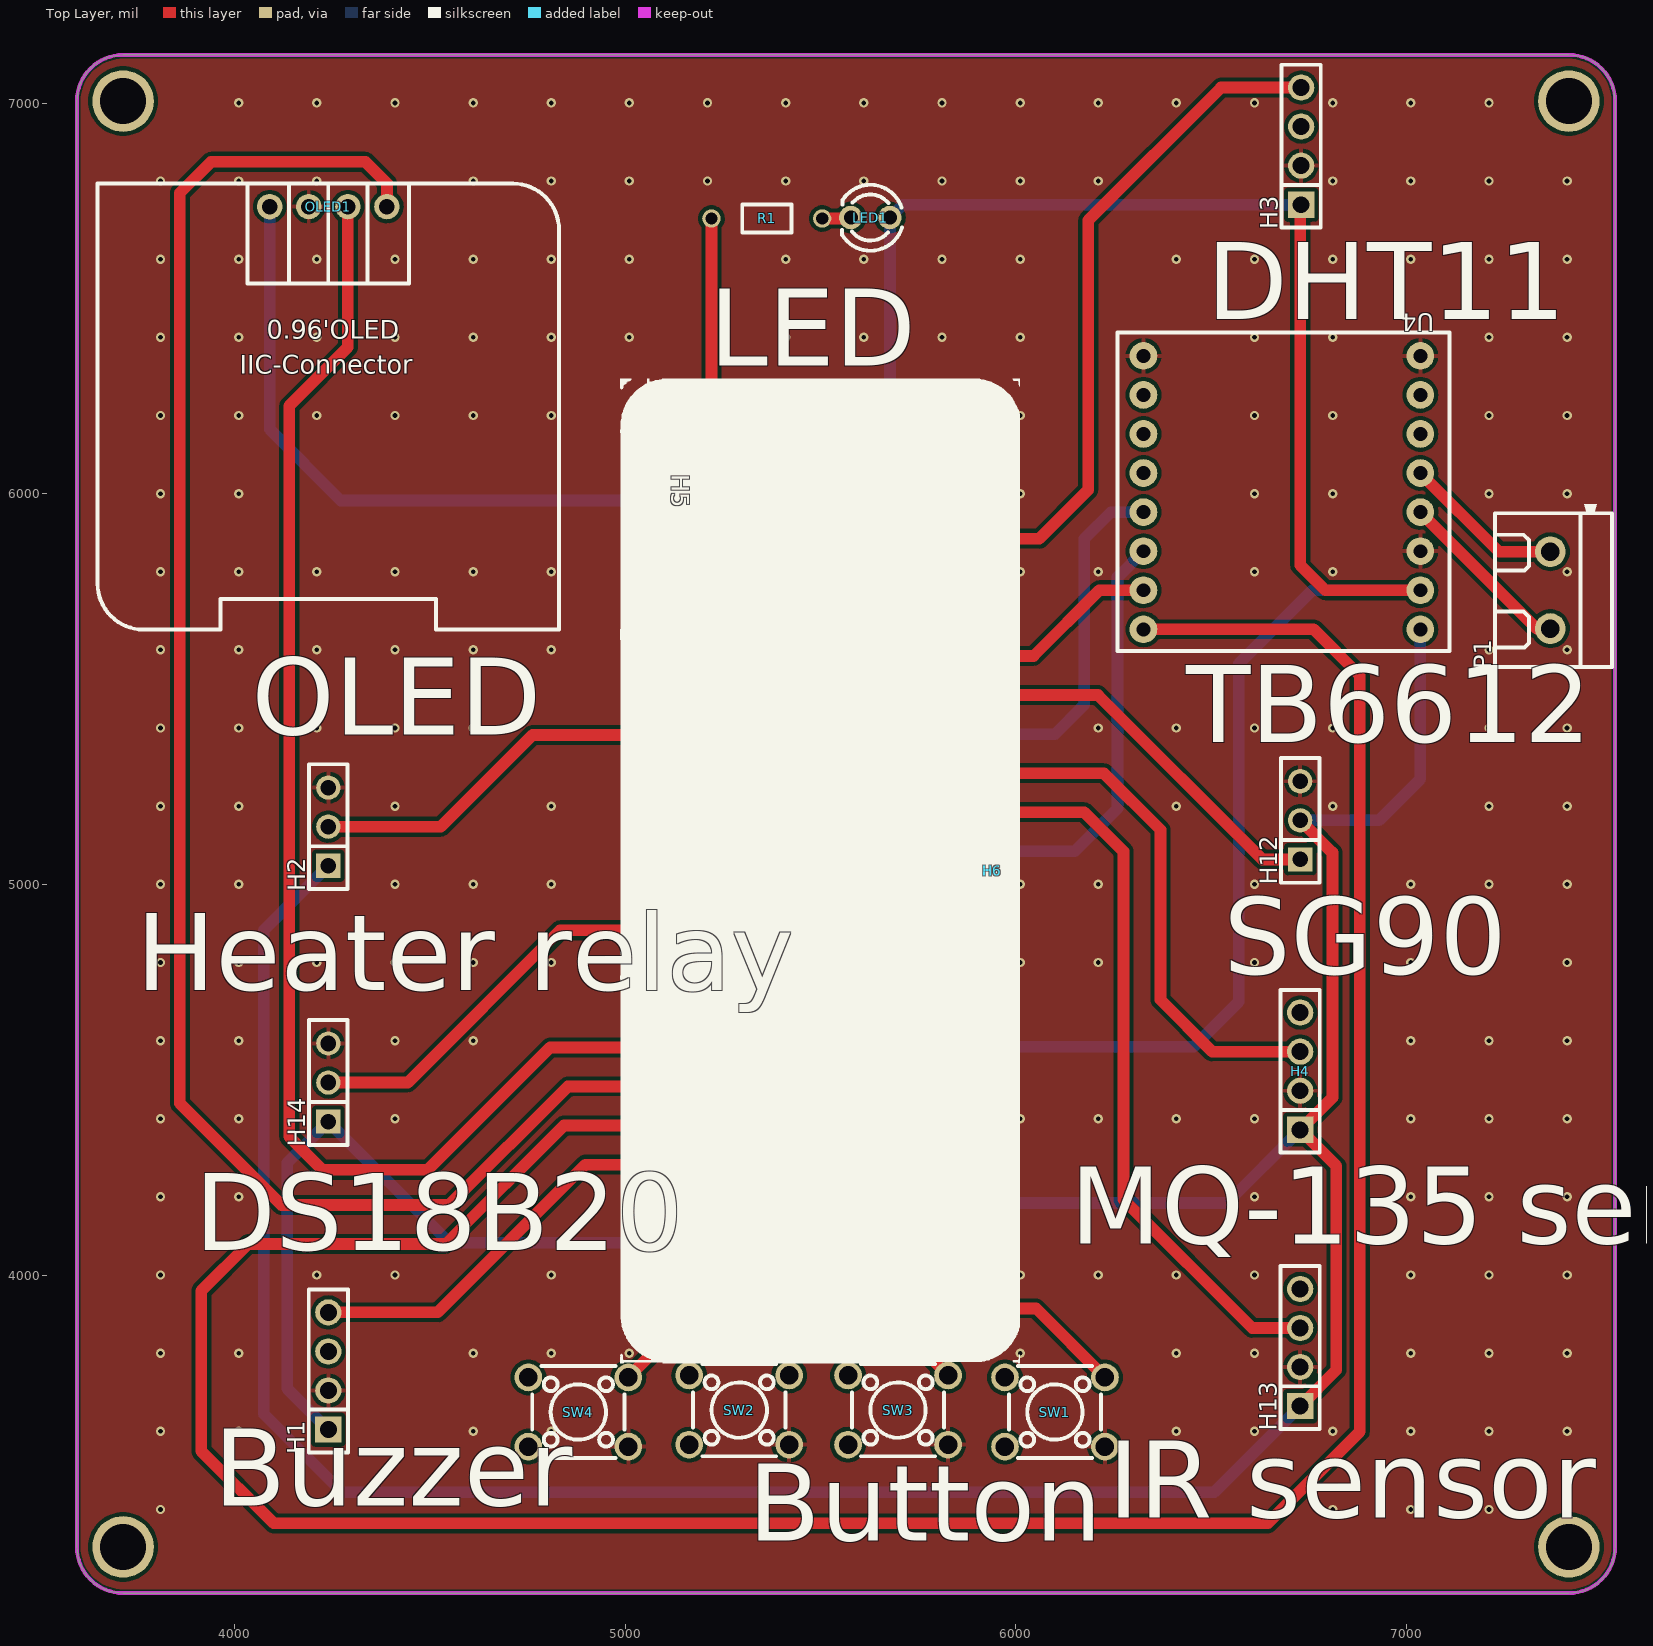
[diagram p0: Top Layer view]
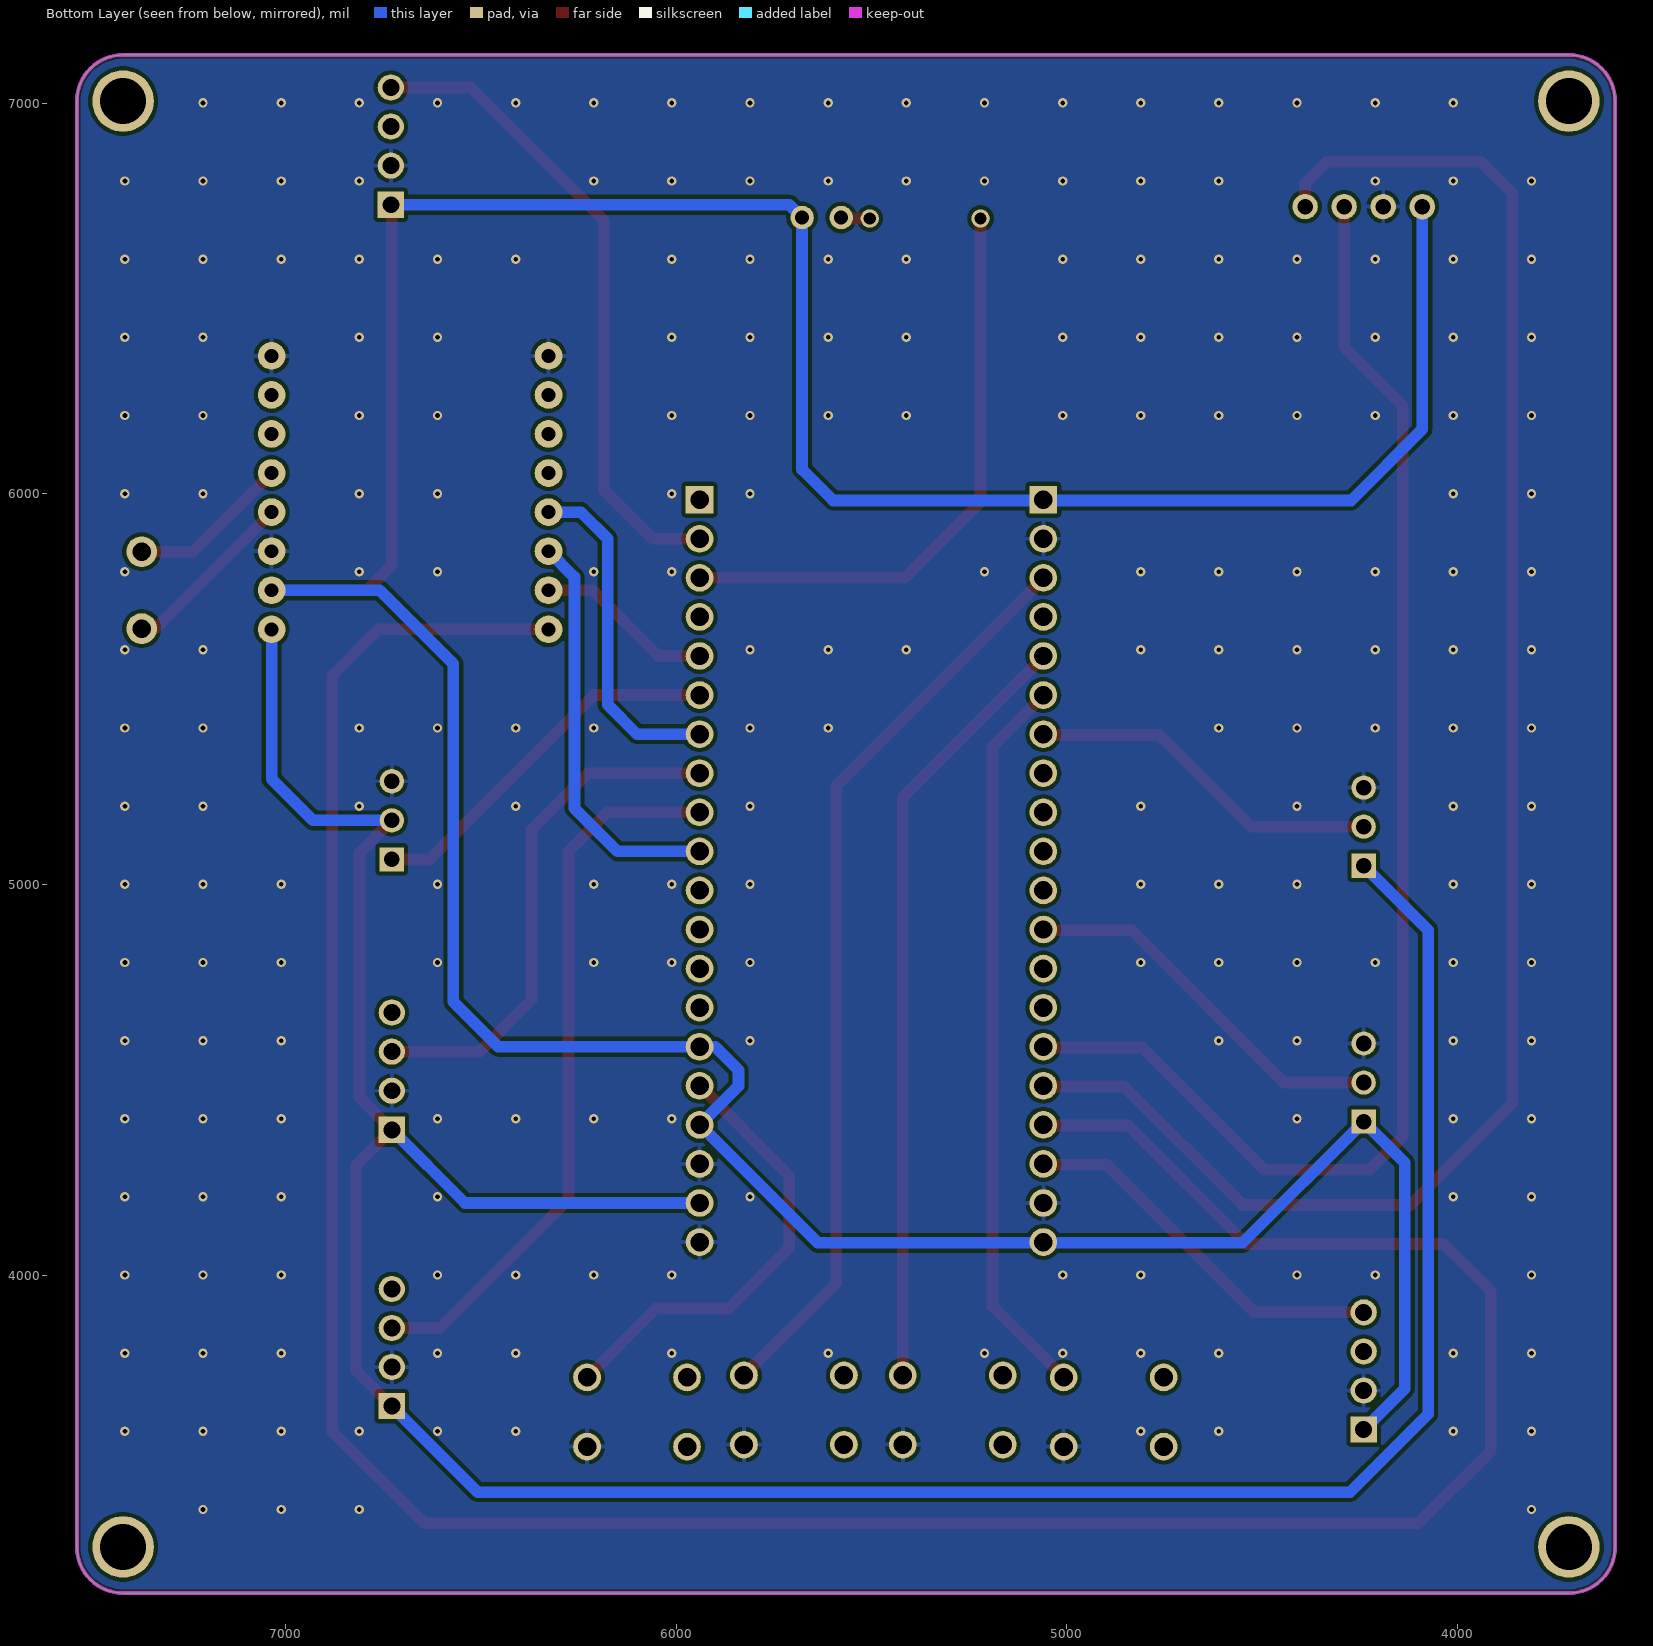
[diagram p1: Bottom Layer view, seen from below]
# Altium PCB MISC89119.pcbdoc
Units mil, origin at the board's own origin, x right, y up, seen from the top; angles counter-clockwise.
Board outline 3937.01 x 3937.01 mil, 2 copper layers (Top Layer, Bottom Layer), stack 62.206 mil thick; 18 components, 37 nets, 111 pads, 222 vias.

## Layer stack, top to bottom
Top Solder Mask Layer: solder mask 0.394, Dk 3.3
Top Layer: signal copper 1.379
Dielectric1: surface 59.449, FR4, Dk 4.5
Bottom Layer: signal copper 1.378
Bottom Solder Mask Layer: solder mask 0.394, Dk 3.3

## Board outline
3714.61,7123.5 ccw(c3714.61,7005.39) 3596.5,7005.39 3596.5,3304.61 ccw(c3714.61,3304.61) 3714.61,3186.5 7415.39,3186.5 ccw(c7415.39,3304.61) 7533.5,3304.61 7533.5,7005.39 ccw(c7415.39,7005.39) 7415.39,7123.5 3714.61,7123.5

## Design rules (kind name [scope] priority, off if disabled: settings)
BoardOutlineClearance copperThickness2oz_1 [All] p2 off: genericclearance=7.99 ignorepadtopadclearanceinfootprint=FALSE except(0: Arc-SplitContinuation Track-SplitContinuation SMDPad-SplitContinuation THPad-SplitContinuation Via-SplitContinuation Fill-SplitContinuation Region-SplitContinuation Poly-SplitContinuation Text-SplitContinuation Hole-SplitContinuation; 5.98: Arc-CutoutEdge Track-CutoutEdge SMDPad-CutoutEdge THPad-CutoutEdge Via-CutoutEdge Text-CutoutEdge; 6.9: Hole-OutlineEdge Hole-CutoutEdge; 10: Poly-OutlineEdge Poly-CutoutEdge; 11.81: Arc-OutlineEdge Track-OutlineEdge SMDPad-OutlineEdge THPad-OutlineEdge Via-OutlineEdge Fill-OutlineEdge Region-OutlineEdge Text-OutlineEdge Fill-CutoutEdge Region-CutoutEdge)
BoardOutlineClearance Plane_innerPlane_1 [All] p4 off: genericclearance=4.02 ignorepadtopadclearanceinfootprint=FALSE except(0: Arc-SplitContinuation Track-SplitContinuation SMDPad-SplitContinuation THPad-SplitContinuation Via-SplitContinuation Fill-SplitContinuation Region-SplitContinuation Poly-SplitContinuation Text-SplitContinuation Hole-SplitContinuation; 5.98: Arc-CutoutEdge Track-CutoutEdge SMDPad-CutoutEdge THPad-CutoutEdge Via-CutoutEdge Text-CutoutEdge; 6.9: Hole-OutlineEdge Hole-CutoutEdge; 10: Poly-OutlineEdge Poly-CutoutEdge; 11.81: Arc-OutlineEdge Track-OutlineEdge SMDPad-OutlineEdge THPad-OutlineEdge Via-OutlineEdge Fill-OutlineEdge Region-OutlineEdge Text-OutlineEdge Fill-CutoutEdge Region-CutoutEdge)
BoardOutlineClearance Copper_copperRegion_1 [All] p6 off: genericclearance=4.02 ignorepadtopadclearanceinfootprint=FALSE except(0: Arc-SplitContinuation Track-SplitContinuation SMDPad-SplitContinuation THPad-SplitContinuation Via-SplitContinuation Fill-SplitContinuation Region-SplitContinuation Poly-SplitContinuation Text-SplitContinuation Hole-SplitContinuation; 5.98: Arc-CutoutEdge Track-CutoutEdge SMDPad-CutoutEdge THPad-CutoutEdge Via-CutoutEdge Text-CutoutEdge; 6.9: Hole-OutlineEdge Hole-CutoutEdge; 10: Poly-OutlineEdge Poly-CutoutEdge; 11.81: Arc-OutlineEdge Track-OutlineEdge SMDPad-OutlineEdge THPad-OutlineEdge Via-OutlineEdge Fill-OutlineEdge Region-OutlineEdge Text-OutlineEdge Fill-CutoutEdge Region-CutoutEdge)
BoardOutlineClearance Copper_copperRegion_copperThickness1oz_1 [All] p8 off: genericclearance=4.02 ignorepadtopadclearanceinfootprint=FALSE except(0: Arc-SplitContinuation Track-SplitContinuation SMDPad-SplitContinuation THPad-SplitContinuation Via-SplitContinuation Fill-SplitContinuation Region-SplitContinuation Poly-SplitContinuation Text-SplitContinuation Hole-SplitContinuation; 5.98: Arc-CutoutEdge Track-CutoutEdge SMDPad-CutoutEdge THPad-CutoutEdge Via-CutoutEdge Text-CutoutEdge; 6.9: Hole-OutlineEdge Hole-CutoutEdge; 10: Poly-OutlineEdge Poly-CutoutEdge; 11.81: Arc-OutlineEdge Track-OutlineEdge SMDPad-OutlineEdge THPad-OutlineEdge Via-OutlineEdge Fill-OutlineEdge Region-OutlineEdge Text-OutlineEdge Fill-CutoutEdge Region-CutoutEdge)
BoardOutlineClearance Copper_copperRegion_Copper_copperRegion_1 [All] p10 off: genericclearance=4.02 ignorepadtopadclearanceinfootprint=FALSE except(0: Arc-SplitContinuation Track-SplitContinuation SMDPad-SplitContinuation THPad-SplitContinuation Via-SplitContinuation Fill-SplitContinuation Region-SplitContinuation Poly-SplitContinuation Text-SplitContinuation Hole-SplitContinuation; 5.98: Arc-CutoutEdge Track-CutoutEdge SMDPad-CutoutEdge THPad-CutoutEdge Via-CutoutEdge Text-CutoutEdge; 6.9: Hole-OutlineEdge Hole-CutoutEdge; 10: Poly-OutlineEdge Poly-CutoutEdge; 11.81: Arc-OutlineEdge Track-OutlineEdge SMDPad-OutlineEdge THPad-OutlineEdge Via-OutlineEdge Fill-OutlineEdge Region-OutlineEdge Text-OutlineEdge Fill-CutoutEdge Region-CutoutEdge)
BoardOutlineClearance copperThickness1oz_1 [All] p12: genericclearance=4.02 ignorepadtopadclearanceinfootprint=FALSE except(0: Arc-SplitContinuation Track-SplitContinuation SMDPad-SplitContinuation THPad-SplitContinuation Via-SplitContinuation Fill-SplitContinuation Region-SplitContinuation Poly-SplitContinuation Text-SplitContinuation Hole-SplitContinuation; 5.98: Arc-CutoutEdge Track-CutoutEdge SMDPad-CutoutEdge THPad-CutoutEdge Via-CutoutEdge Text-CutoutEdge; 6.9: Hole-OutlineEdge Hole-CutoutEdge; 10: Poly-OutlineEdge Poly-CutoutEdge; 11.81: Arc-OutlineEdge Track-OutlineEdge SMDPad-OutlineEdge THPad-OutlineEdge Via-OutlineEdge Fill-OutlineEdge Region-OutlineEdge Text-OutlineEdge Fill-CutoutEdge Region-CutoutEdge)
Clearance copperThickness2oz [All] p1 off: gap=7.99 ignorepadtopadclearanceinfootprint=FALSE except(5.98: SMDPad-Track SMDPad-SMDPad THPad-Track SMDPad-THPad THPad-THPad Track-Via SMDPad-Via THPad-Via Via-Via Fill-SMDPad Region-SMDPad Fill-THPad Region-THPad Fill-Via Region-Via Fill-Fill Fill-Region Region-Region Arc-Track Arc-SMDPad Arc-THPad Arc-Via Fill-Arc Region-Arc Arc-Arc Text-Track SMDPad-Text Text-THPad Text-Via Fill-Text Region-Text Arc-Text Text-Text; 6.9: Hole-Track Hole-SMDPad Hole-THPad Hole-Via Fill-Hole Region-Hole Hole-Arc Hole-Text; 10: Poly-Track Poly-SMDPad Poly-THPad Poly-Via Poly-Fill Poly-Region Poly-Poly Poly-Arc Poly-Text Poly-Hole; 11.81: Fill-Track Region-Track)
Clearance Plane_innerPlane [All] p3 off: gap=4.02 ignorepadtopadclearanceinfootprint=FALSE except(5.98: SMDPad-Track SMDPad-SMDPad THPad-Track SMDPad-THPad THPad-THPad Track-Via SMDPad-Via THPad-Via Via-Via Fill-SMDPad Region-SMDPad Fill-THPad Region-THPad Fill-Via Region-Via Fill-Fill Fill-Region Region-Region Arc-Track Arc-SMDPad Arc-THPad Arc-Via Fill-Arc Region-Arc Arc-Arc Text-Track SMDPad-Text Text-THPad Text-Via Fill-Text Region-Text Arc-Text Text-Text; 6.9: Hole-Track Hole-SMDPad Hole-THPad Hole-Via Fill-Hole Region-Hole Hole-Arc Hole-Text; 10: Poly-Track Poly-SMDPad Poly-THPad Poly-Via Poly-Fill Poly-Region Poly-Poly Poly-Arc Poly-Text Poly-Hole; 11.81: Fill-Track Region-Track)
Clearance Copper_copperRegion [All] p5 off: gap=4.02 ignorepadtopadclearanceinfootprint=FALSE except(5.98: SMDPad-Track SMDPad-SMDPad THPad-Track SMDPad-THPad THPad-THPad Track-Via SMDPad-Via THPad-Via Via-Via Fill-SMDPad Region-SMDPad Fill-THPad Region-THPad Fill-Via Region-Via Fill-Fill Fill-Region Region-Region Arc-Track Arc-SMDPad Arc-THPad Arc-Via Fill-Arc Region-Arc Arc-Arc Text-Track SMDPad-Text Text-THPad Text-Via Fill-Text Region-Text Arc-Text Text-Text; 6.9: Hole-Track Hole-SMDPad Hole-THPad Hole-Via Fill-Hole Region-Hole Hole-Arc Hole-Text; 10: Poly-Track Poly-SMDPad Poly-THPad Poly-Via Poly-Fill Poly-Region Poly-Poly Poly-Arc Poly-Text Poly-Hole; 11.81: Fill-Track Region-Track)
Clearance Copper_copperRegion_copperThickness1oz [All] p7 off: gap=4.02 ignorepadtopadclearanceinfootprint=FALSE except(5.98: SMDPad-Track SMDPad-SMDPad THPad-Track SMDPad-THPad THPad-THPad Track-Via SMDPad-Via THPad-Via Via-Via Fill-SMDPad Region-SMDPad Fill-THPad Region-THPad Fill-Via Region-Via Fill-Fill Fill-Region Region-Region Arc-Track Arc-SMDPad Arc-THPad Arc-Via Fill-Arc Region-Arc Arc-Arc Text-Track SMDPad-Text Text-THPad Text-Via Fill-Text Region-Text Arc-Text Text-Text; 6.9: Hole-Track Hole-SMDPad Hole-THPad Hole-Via Fill-Hole Region-Hole Hole-Arc Hole-Text; 10: Poly-Track Poly-SMDPad Poly-THPad Poly-Via Poly-Fill Poly-Region Poly-Poly Poly-Arc Poly-Text Poly-Hole; 11.81: Fill-Track Region-Track)
Clearance Copper_copperRegion_Copper_copperRegion [All] p9 off: gap=4.02 ignorepadtopadclearanceinfootprint=FALSE except(5.98: SMDPad-Track SMDPad-SMDPad THPad-Track SMDPad-THPad THPad-THPad Track-Via SMDPad-Via THPad-Via Via-Via Fill-SMDPad Region-SMDPad Fill-THPad Region-THPad Fill-Via Region-Via Fill-Fill Fill-Region Region-Region Arc-Track Arc-SMDPad Arc-THPad Arc-Via Fill-Arc Region-Arc Arc-Arc Text-Track SMDPad-Text Text-THPad Text-Via Fill-Text Region-Text Arc-Text Text-Text; 6.9: Hole-Track Hole-SMDPad Hole-THPad Hole-Via Fill-Hole Region-Hole Hole-Arc Hole-Text; 10: Poly-Track Poly-SMDPad Poly-THPad Poly-Via Poly-Fill Poly-Region Poly-Poly Poly-Arc Poly-Text Poly-Hole; 11.81: Fill-Track Region-Track)
Clearance copperThickness1oz [All] p11: gap=4.02 ignorepadtopadclearanceinfootprint=FALSE except(5.98: SMDPad-Track SMDPad-SMDPad THPad-Track SMDPad-THPad THPad-THPad Track-Via SMDPad-Via THPad-Via Via-Via Fill-SMDPad Region-SMDPad Fill-THPad Region-THPad Fill-Via Region-Via Fill-Fill Fill-Region Region-Region Arc-Track Arc-SMDPad Arc-THPad Arc-Via Fill-Arc Region-Arc Arc-Arc Text-Track SMDPad-Text Text-THPad Text-Via Fill-Text Region-Text Arc-Text Text-Text; 6.9: Hole-Track Hole-SMDPad Hole-THPad Hole-Via Fill-Hole Region-Hole Hole-Arc Hole-Text; 10: Poly-Track Poly-SMDPad Poly-THPad Poly-Via Poly-Fill Poly-Region Poly-Poly Poly-Arc Poly-Text Poly-Hole; 11.81: Fill-Track Region-Track)
DiffPairsRouting differentialPair [All] p1: maxlimit=6 minlimit=6 mostfreqgap=6 toplayer_minwidth=5 toplayer_prefwidth=10 toplayer_maxwidth=100 toplayer_mingap=6 toplayer_prefgap=6 toplayer_maxgap=6 bottomlayer_minwidth=5 bottomlayer_prefwidth=10 bottomlayer_maxwidth=100 bottomlayer_mingap=6 bottomlayer_prefgap=6 bottomlayer_maxgap=6 maxuncoupledlength=10
HoleToHoleClearance otherClearance [All] p1: gap=11.81 allowstackedmicrovias=TRUE
Length netLength [All] p1: minlimit=0 maxlimit=0
PasteMaskExpansion pasteMaskExpansion [All] p1: expansion=0
PlaneConnect innerPlane [All] p1: planeconnectstyle=Relief reliefexpansion=20 reliefentries=4 reliefconductorwidth=10 reliefairgap=10
PolygonConnect copperRegion_copperThickness1oz [All] p1 off: connectstyle=Relief reliefconductorwidth=10 reliefentries=4 polygonreliefangle="90 Angle" airgapwidth=10 via.connectstyle=Relief via.reliefconductorwidth=10 via.reliefentries=4 via.polygonreliefangle="90 Angle" via.airgapwidth=10
PolygonConnect copperRegion_Copper_copperRegion [All] p2 off: connectstyle=Relief reliefconductorwidth=10 reliefentries=4 polygonreliefangle="90 Angle" airgapwidth=10 via.connectstyle=Relief via.reliefconductorwidth=10 via.reliefentries=4 via.polygonreliefangle="90 Angle" via.airgapwidth=10
PolygonConnect copperRegion [All] p3: connectstyle=Relief reliefconductorwidth=10 reliefentries=4 polygonreliefangle="90 Angle" airgapwidth=10 via.connectstyle=Relief via.reliefconductorwidth=10 via.reliefentries=4 via.polygonreliefangle="90 Angle" via.airgapwidth=10
RoutingVias viaSize [All] p1: holewidth=12.01 width=24.02 viastyle="Through Hole" minholewidth=11.81 minwidth=19.68 maxholewidth=248.03 maxwidth=393.7
SolderMaskExpansion solderMaskExpansion [IsVia] p1: expansion=-1000 istentingtop=TRUE
SolderMaskExpansion solderMaskExpansion [All] p2: expansion=2 istentingtop=FALSE
Width copperThickness2oz_2 [All] p1 off: maxlimit=100 minlimit=8 preferedwidth=10
Width copperThickness1oz_2 [All] p2: maxlimit=100 minlimit=5 preferedwidth=10

## Components (designator, comment, footprint, x,y, rotation, side; value= is the part's Value field where it differs from the comment)
H1 "" HDR-TH_4P-P2.54-V-F 4240,3755 r90 top
H2 "" HDR-TH_3P-P2.54-V-F 4240,5148.1 r90 top
H3 "" HDR-TH_4P-P2.54-V-F 6730,6890 r90 top
H4 "" HDR-TH_4P-P2.54-V-F 6727.5,4522.29 r90 top
H5 "" HDR-TH_20P-P2.54-V-F 5060,5035 r270 top
H6 "" HDR-TH_20P-P2.54-V-F 5939.74,5034.94 r270 top
H12 "" HDR-TH_3P-P2.54-V-F 6727.5,5164.4 r90 top
H13 "" HDR-TH_4P-P2.54-V-F 6727.5,3815.05 r90 top
H14 "" HDR-TH_3P-P2.54-V-F 4240,4493.24 r90 top
LED1 "" LED_TH-3mm 5627.35,6707.23 r180 top
OLED1 "" 0.96OLED_4P 4240,6735 r0 top
P1 "KF301-2P terminal block" CONN-TH_XY301V-A-5.0-2P 7367.76,5753.51 r90 top
R1 "220Ω" Res_1/8W 5362.36,6707.23 r180 top
SW1 "" SW-TH_4P-L6.0-W6.0-P4.50-LS6.5 6099.85,3650 r180 top
SW2 "" SW-TH_4P-L6.0-W6.0-P4.50-LS6.5 5291.62,3655 r180 top
SW3 "" SW-TH_4P-L6.0-W6.0-P4.50-LS6.5 5698.23,3655 r180 top
SW4 "" SW-TH_4P-L6.0-W6.0-P4.50-LS6.5 4880,3650 r180 top
U4 "" tb6612 7035,5653.24 r180 top

## Footprints (in the part's own frame and the unit in brackets; to place one, negate y for a bottom-side part, rotate by r counter-clockwise, add the part's x,y. Pads: shape width x height; smd on the part's side, far side on the other; paste and mask are expansions set on the pad)
0.96OLED_4P [mm]
  round 1.65 hole 1 copper offset 0,0: 1(-3.81,-0.001) 2(-1.27,0.002) 3(1.27,0.002) 4(3.81,0.002)
  silkscreen extent -15,-27.5 15,1.5
CONN-TH_XY301V-A-5.0-2P [mm]
  round 2 hole 1.2: 1(-2.5,0) 2(2.5,0)
  silkscreen extent -5,-4 5.6,3.6
HDR-TH_3P-P2.54-V-F [mil]
  rect 62x62 hole 40.16: 1(-100,0)
  round 62 hole 40.16: 2(0,0) 3(100,0)
  silkscreen extent -160,-49 160,49
HDR-TH_4P-P2.54-V-F [mm]
  rect 1.7x1.7 hole 1.1: 1(-3.81,0)
  round 1.7 hole 1.1: 2(-1.27,0) 3(1.27,0) 4(3.81,0)
  silkscreen extent -5.29,-1.27 5.29,1.27
HDR-TH_20P-P2.54-V-F [mm]
  rect 1.8x1.8 hole 1.2: 1(-24.13,0)
  round 1.8 hole 1.2: 2(-21.59,0) 3(-19.05,0) 4(-16.51,0) 5(-13.97,0) 6(-11.43,0) 7(-8.89,0) 8(-6.35,0) 9(-3.81,0) 10(-1.27,0) 11(1.27,0) 12(3.81,0) 13(6.35,0) 14(8.89,0) 15(11.43,0) 16(13.97,0) 17(16.51,0) 18(19.05,0) 19(21.59,0) 20(24.13,0)
  silkscreen extent -25.65,-1.25 25.65,1.25
LED_TH-3mm [mil]
  round 60 hole 36 paste+0 mask+2: 1(-50,0) 2(50,0)
  silkscreen extent -81,-84 72,85
Res_1/8W [mil]
  round 47.2 hole 31.5 paste+0 mask+2: 1(-141.7,2.48) 2(141.7,2.48)
  silkscreen extent -63,-33 63,38
SW-TH_4P-L6.0-W6.0-P4.50-LS6.5 [mm]
  round 1.8 hole 1.2: 1(-3.25,2.25) 2(3.25,2.25) 3(-3.25,-2.25) 4(3.25,-2.25)
  silkscreen extent -3,-3 3,3
tb6612 [mm]
  round 1.8 hole 0.9: 1(0,0) 2(0,-2.54) 3(0,-5.08) 4(0,-7.62) 5(0,-10.16) 6(0,-12.7) 7(0,-15.24) 8(0,-17.78) 9(18,-17.78) 10(18,-15.24) 11(18,-12.7) 12(18,-10.16) 13(18,-7.62) 14(18,-5.08) 15(18,-2.54) 16(18,0)
  silkscreen extent -1.91,-19.3 19.69,1.4

## Free pads (board coordinates)
  round 157.48 hole 118.11: 1(3714.61,7005.39) 1(3714.61,3304.61) 1(7415.39,7005.39) 1(7415.39,3304.61)

## Via types
v1: diameter 24.02, hole 12, Top Layer to Bottom Layer, 222 vias

## Nets (pads, with @x,y where several pads share a name; then routed paths per layer and width w, separated by ;. In a path a pad name is that pad's centre, name@x,y a point inside that pad or via, vN(x,y) a via of type N, cw(c..) or ccw(c..) an arc to the next point about the centre after c; other vN are vias at no path point)
$1N17195: LED1.2 R1.1 | length 74.3
  Top Layer w30: R1.1 5574.87,6704.75 LED1.2
$1N17231: P1.1 U4.4 | length 456.3
  Top Layer w30: U4.4 7333.15,5655.09 P1.1
$1N17232: P1.2 U4.5 | length 416.1
  Top Layer w30: U4.5 7236.3,5851.94 P1.2
+5V: H2.1 H4.1 H6.19 H12.2 H13.1 U4.1 | length 7542.1
  Top Layer w30: H13.1 6820,3757.55 6820,4279.79 H4.1 6810,4454.79 6810,5081.9 H12.2
  Bottom Layer w30: H2.1 4075,4883.1 4075,3645 4275,3445 6507.45,3445 H13.1 ; H6.19 6540.15,4184.94 H4.1 ; H12.2 6929.4,5164.4 7035,5270 U4.1
A0: H6.14
A1: H6.13
A2: H6.12
A3: H6.11
A4: H6.10 U4.14 | length 1051.6
  Bottom Layer w30: H6.10 6149.94,5084.94 6260,5195 6260,5786.91 U4.14
A5: H6.9 H13.3 | length 1855.8
  Top Layer w30: H6.9 6175.06,5184.94 6275,5085 6275,4195 6604.95,3865.05 H13.3
A6: H4.3 H6.8 | length 1337.8
  Top Layer w30: H6.8 6225.06,5284.94 6370,5140 6370,4705 6502.71,4572.29 H4.3
A7: H6.7 U4.13 | length 870.9
  Bottom Layer w30: H6.7 6099.94,5384.94 6175,5460 6175,5885 6243.24,5953.24 U4.13
A8: H2.2 H5.7 | length 917.1
  Top Layer w30: H2.2 4528.1,5148.1 4763.05,5383.05 H5.7@5059.74,5383.05
A9: H5.5 SW2.3 | length 1988.5
  Top Layer w30: H5.5@5059.74,5583.05 5419.57,5223.22 SW2.3
A10: H5.6 SW4.3 | length 1873.8
  Top Layer w30: SW4.3 5190,3920.63 5190,5352.79 H5.6@5059.74,5483.05
A11: H5.3 SW3.3 | length 2356.9
  Top Layer w30: H5.3@5059.74,5783.05 5590,5252.79 5590,3979.76 SW3.3
A12: H5.4
A15: H5.11
B0: H6.6 H12.1 | length 962
  Top Layer w30: H6.6 6210.06,5484.94 6630.6,5064.4 H12.1
B1: H6.5 U4.15 | length 456.3
  Top Layer w30: H6.5 6044.94,5584.94 6213.24,5753.24 U4.15
B3: H5.12 H14.2 | length 981.2
  Top Layer w30: H14.2 4443.24,4493.24 4833.05,4883.05 H5.12@5059.74,4883.05
B4: H5.13
B5: H5.14
B6: H5.15 OLED1.3 | length 3526.8
  Top Layer w30: OLED1.3@4290,6735.05 4290,6375 4140,6225 4140,4355 4225,4270 4495,4270 4808.05,4583.05 H5.15@5059.74,4583.05
B7: H5.16 OLED1.4 | length 4408.8
  Top Layer w30: OLED1.4@4390,6735.05 4390,6795 4335,6850 3940,6850 3860,6770 3860,4440 4120,4180 4550,4180 4853.05,4483.05 H5.16@5059.74,4483.05
B8: H5.17 U4.16 | length 7406.6
  Top Layer w30: H5.17@5059.74,4383.05 4843.05,4383.05 4540,4080 4035,4080 3915,3960 3915,3550 4100,3365 6645,3365 6880,3600 6880,5535 6761.76,5653.24 U4.16
B9: H1.4 H5.18 | length 976.3
  Top Layer w30: H1.4 4520,3905 4898.05,4283.05 H5.18@5059.74,4283.05
B10: H6.4
B11: H6.3 R1.2 | length 1525
  Top Layer w30: R1.2 5220.66,5979.34 5415.06,5784.94 H6.3
B12: H3.4 H6.2 | length 1672.9
  Top Layer w30: H6.2 6059.94,5884.94 6185,6010 6185,6700 6525,7040 H3.4
B13: H5.10
B14: H5.9
B15: H5.8
C13: H6.16 SW1.3 | length 1165.2
  Top Layer w30: H6.16 5710,4255.2 5710,4070 5865,3915 6051.38,3915 SW1.3
GND: H1.2 H2.3 H3.2 H4.2 H5.2 H5.19 H6.18 H6.20 H12.3 H13.2 H14.3 OLED1.2 SW1.1 SW2.1 SW3.1 SW4.1 U4.3 U4.8 U4.9
  other v1: 3810.6,3400.6 6810.6,3400.6 7010.6,3400.6 7210.6,3400.6 3810.6,3600.6 4010.6,3600.6 4610.6,3600.6 4810.6,3600.6 6410.6,3600.6 6610.6,3600.6 6810.6,3600.6 7010.6,3600.6 7210.6,3600.6 7410.6,3600.6 3810.6,3800.6 4010.6,3800.6 4610.6,3800.6 4810.6,3800.6 5010.6,3800.6 5210.6,3800.6 5610.6,3800.6 6010.6,3800.6 6410.6,3800.6 6610.6,3800.6 7010.6,3800.6 7210.6,3800.6 7410.6,3800.6 3810.6,4000.6 4210.6,4000.6 4410.6,4000.6 4810.6,4000.6 5010.6,4000.6 6010.6,4000.6 6210.6,4000.6 6410.6,4000.6 6610.6,4000.6 7010.6,4000.6 7210.6,4000.6 7410.6,4000.6 3810.6,4200.6 4010.6,4200.6 5810.6,4200.6 6610.6,4200.6 7010.6,4200.6 7210.6,4200.6 7410.6,4200.6 3810.6,4400.6 4010.6,4400.6 4410.6,4400.6 6010.6,4400.6 6210.6,4400.6 6410.6,4400.6 6610.6,4400.6 7010.6,4400.6 7210.6,4400.6 7410.6,4400.6 3810.6,4600.6 4010.6,4600.6 4410.6,4600.6 4610.6,4600.6 5810.6,4600.6 7010.6,4600.6 7210.6,4600.6 7410.6,4600.6 3810.6,4800.6 4010.6,4800.6 4210.6,4800.6 4410.6,4800.6 4610.6,4800.6 4810.6,4800.6 5810.6,4800.6 6010.6,4800.6 6210.6,4800.6 6610.6,4800.6 7010.6,4800.6 7210.6,4800.6 7410.6,4800.6 3810.6,5000.6 4010.6,5000.6 4410.6,5000.6 4610.6,5000.6 4810.6,5000.6 5810.6,5000.6 6010.6,5000.6 6210.6,5000.6 6610.6,5000.6 7010.6,5000.6 7210.6,5000.6 7410.6,5000.6 3810.6,5200.6 4010.6,5200.6 4410.6,5200.6 4810.6,5200.6 5810.6,5200.6 6410.6,5200.6 6810.6,5200.6 7210.6,5200.6 7410.6,5200.6 3810.6,5400.6 4010.6,5400.6 4210.6,5400.6 4410.6,5400.6 4610.6,5400.6 5610.6,5400.6 5810.6,5400.6 6210.6,5400.6 6410.6,5400.6 6610.6,5400.6 6810.6,5400.6 7210.6,5400.6 7410.6,5400.6 3810.6,5600.6 4010.6,5600.6 4210.6,5600.6 4410.6,5600.6 4610.6,5600.6 4810.6,5600.6 5410.6,5600.6 5610.6,5600.6 5810.6,5600.6 7210.6,5600.6 7410.6,5600.6 3810.6,5800.6 4010.6,5800.6 4210.6,5800.6 4410.6,5800.6 4610.6,5800.6 4810.6,5800.6 5210.6,5800.6 6010.6,5800.6 6210.6,5800.6 6610.6,5800.6 6810.6,5800.6 7410.6,5800.6 3810.6,6000.6 4010.6,6000.6 5810.6,6000.6 6010.6,6000.6 6610.6,6000.6 6810.6,6000.6 7210.6,6000.6 7410.6,6000.6 3810.6,6200.6 4010.6,6200.6 4210.6,6200.6 4410.6,6200.6 4610.6,6200.6 4810.6,6200.6 5010.6,6200.6 5410.6,6200.6 5610.6,6200.6 5810.6,6200.6 6010.6,6200.6 6610.6,6200.6 6810.6,6200.6 7210.6,6200.6 7410.6,6200.6 3810.6,6400.6 4010.6,6400.6 4210.6,6400.6 4410.6,6400.6 4610.6,6400.6 4810.6,6400.6 5010.6,6400.6 5410.6,6400.6 5610.6,6400.6 5810.6,6400.6 6010.6,6400.6 6610.6,6400.6 6810.6,6400.6 7210.6,6400.6 7410.6,6400.6 3810.6,6600.6 4010.6,6600.6 4210.6,6600.6 4410.6,6600.6 4610.6,6600.6 4810.6,6600.6 5010.6,6600.6 5410.6,6600.6 5610.6,6600.6 5810.6,6600.6 6010.6,6600.6 6410.6,6600.6 6610.6,6600.6 6810.6,6600.6 7010.6,6600.6 7210.6,6600.6 7410.6,6600.6 3810.6,6800.6 4010.6,6800.6 4210.6,6800.6 4610.6,6800.6 4810.6,6800.6 5010.6,6800.6 5210.6,6800.6 5410.6,6800.6 5610.6,6800.6 5810.6,6800.6 6010.6,6800.6 6210.6,6800.6 6810.6,6800.6 7010.6,6800.6 7210.6,6800.6 7410.6,6800.6 4010.6,7000.6 4210.6,7000.6 4410.6,7000.6 4610.6,7000.6 4810.6,7000.6 5010.6,7000.6 5210.6,7000.6 5410.6,7000.6 5610.6,7000.6 5810.6,7000.6 6010.6,7000.6 6210.6,7000.6 6410.6,7000.6 6610.6,7000.6 6810.6,7000.6 7010.6,7000.6 7210.6,7000.6
VBAT: H6.1
VCC: H1.1 H3.1 H5.1 H5.20 H6.15 H6.17 H14.1 LED1.1 OLED1.1 U4.2 | length 10451.1
  Top Layer w30: H3.1@6727.5,6740 6727.5,5817.5 6791.76,5753.24 U4.2
  Bottom Layer w30: OLED1.1 4090,6165 4271.95,5983.05 5598.05,5983.05 5677.35,6062.35 LED1.1 5710.12,6740 H3.1@6727.5,6740 ; H1.1 4135,3710 4135,4288.25 H14.1 4550.19,4083.05 5637.85,4083.05 H6.17 5840,4484.68 5840,4525 5899.94,4584.94 H6.15 6454.94,4584.94 6570,4700 6570,5565 6758.24,5753.24 U4.2
pads on no net: H1.3 H3.3 H4.4 H13.4 SW1.2 SW1.4 SW2.2 SW2.4 SW3.2 SW3.4 SW4.2 SW4.4 U4.6 U4.7 U4.10 U4.11 U4.12

## Polygon pours and split planes (outlines as drawn)
GND on Bottom Layer (solid, remove dead copper, pour order 2): 3525,7245 3525,3080 7700,3080 7700,7245
GND on Top Layer (solid, remove dead copper, pour order 2): 3000,7415 3000,3000 7930,3000 7930,7415

## Keep-outs
Board Outline Layer:
  the board outline again, w10

## Silkscreen, mask and mechanical layers (free items; w line width, h text height)
Top Silkscreen Layer:
  drawing of 450 lines, arcs and shapes, not listed
  text "DHT11" at 6488.89,6446.82 h196.85
  text "LED" at 5215.32,6327.95 h196.85
  text "OLED" at 4043.44,5383.51 h196.85
  text "TB6612" at 6435.8,5364.61 h196.85
  text "SG90" at 6531.54,4770.92 h196.85
  text "Heater relay" at 3747.98,4729.25 h196.85
  text "MQ-135 sensor" at 6139.33,4080.38 h196.85
  text "DS18B20" at 3898.04,4064.56 h196.85
  text "Buzzer" at 3946.81,3410 h196.85
  text "IR sensor" at 6235.97,3380 h196.85
  text "Button" at 5315,3320 h196.85